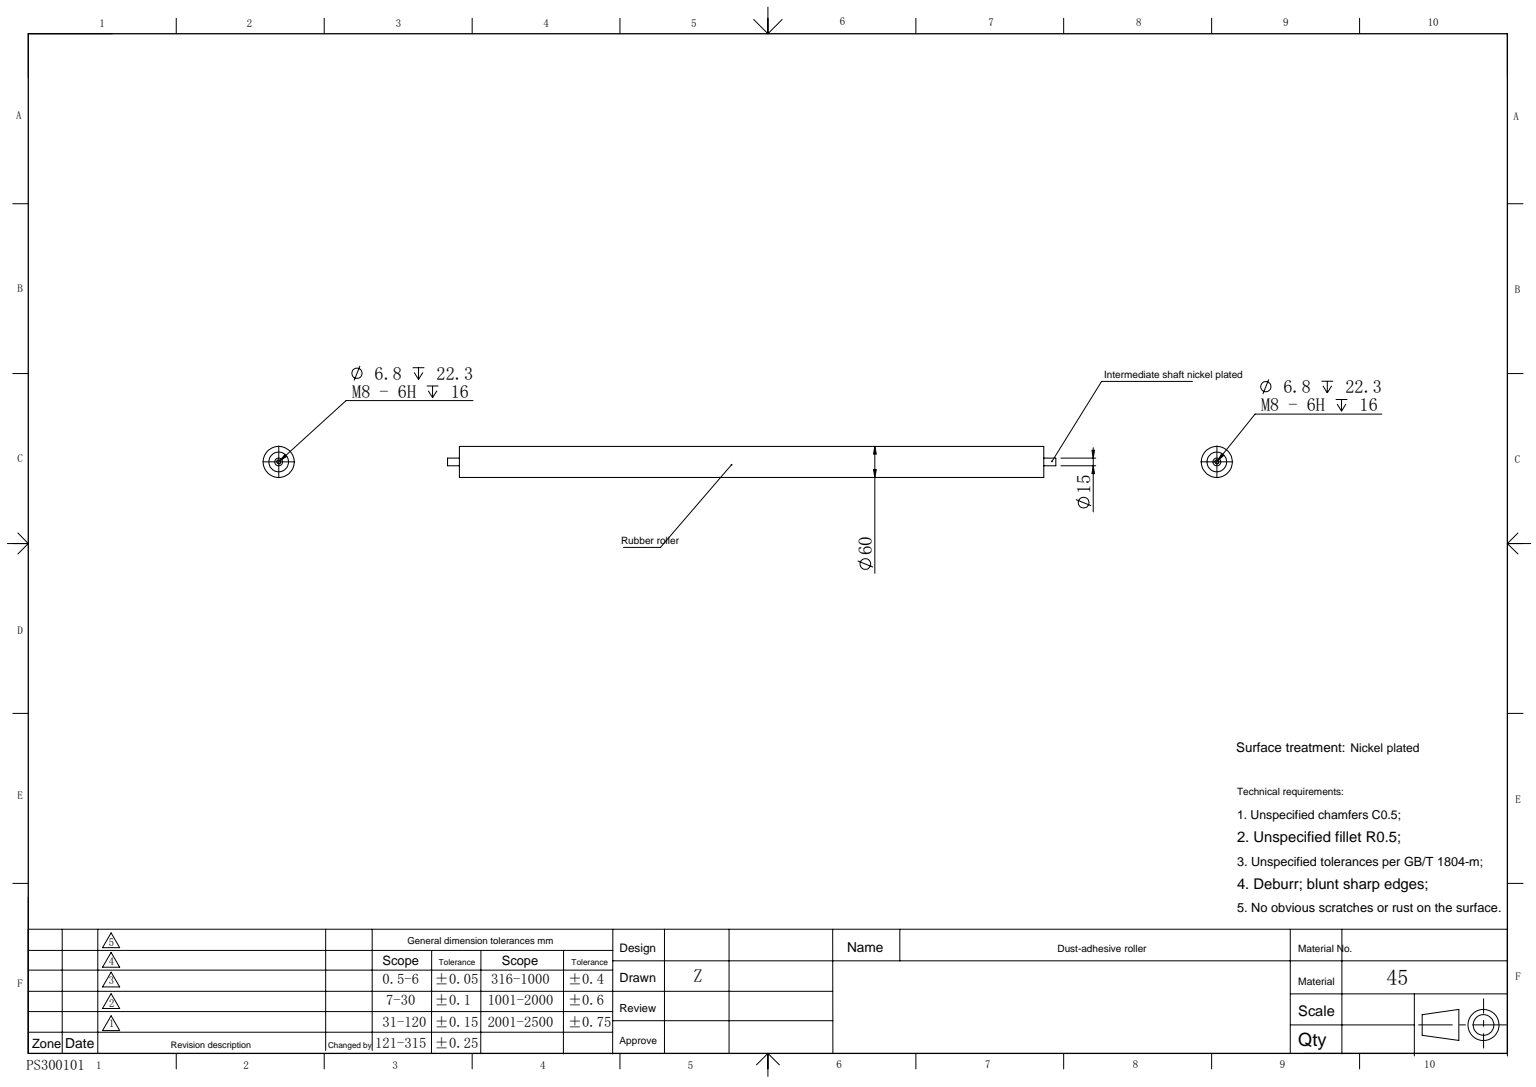
SolidWorks part; units mm, degrees
ref_plane "前视基准面" through (0, 0, 0) normal (0, 0, 1) x (1, 0, 0)
ref_plane "上视基准面" through (0, 0, 0) normal (0, 1, 0) x (1, 0, 0)
ref_plane "右视基准面" through (0, 0, 0) normal (1, 0, 0) x (0, 0, -1)
sketch "草图1" plane through (0, 0, 0) normal (0, 0, 1) x (1, 0, 0)
  circle A0 centre (0, 0) radius 7.5
  dimension "D1" = 15
extrude "凸台-拉伸1" add sketch "草图1" along normal mid plane 1176
sketch "草图2" plane through (0, 0, 0) normal (0, 0, 1) x (1, 0, 0)
  circle A0 centre (0, 0) radius 19
  dimension "D1" = 38
extrude "凸台-拉伸2" add sketch "草图2" along normal mid plane 1100
sketch "草图3" plane through (0, 0, 0) normal (0, 0, 1) x (1, 0, 0)
  circle A0 centre (0, 0) radius 30
  circle A1 centre (0, 0) radius 19
  circle A2 centre (0, 0) radius 19 construction
  dimension "D1" = 60
extrude "凸台-拉伸3" add sketch "草图3" along normal mid plane 1130 separate body
sketch "草图6" plane through (0, 0, -588) normal (0, 0, -1) x (-1, 0, 0)
  point P0 (0, 0)
hole_wizard "M8 螺纹孔1" positions "草图6" profile "草图5" tap size "M8" standard "ISO"
sketch "草图5" plane through (0, 0, -588) normal (1, 0, 0) x (0, 1, 0)
  line L0 (0, 0) -> (0, 24.2929)
  line L1 (0, 24.2929) -> (3.4, 22.25)
  line L2 (3.4, 22.25) -> (3.4, 0)
  line L5 (3.4, 0) -> (0, 0)
  line L10 (0, 24.2929) -> (-3.4, 22.25) construction
  line L11 (0, -6.35) -> (0, 107.95) construction
  dimension "螺纹孔钻头直径" = 6.8
  dimension "螺纹孔钻头深度" = 22.25
  dimension "导头角度" = 118
cosmetic thread "孔螺纹线1" parameters "D1"=16, "D2"=8
sketch "草图9" plane through (0, 0, 588) normal (0, 0, 1) x (1, 0, 0)
  point P0 (0, 0)
hole_wizard "M8 螺纹孔2" positions "草图9" profile "草图8" tap size "M8" standard "ISO"
sketch "草图8" plane through (0, 0, 588) normal (1, 0, 0) x (0, -1, 0)
  line L0 (0, 0) -> (0, 24.2929)
  line L1 (0, 24.2929) -> (3.4, 22.25)
  line L2 (3.4, 22.25) -> (3.4, 0)
  line L5 (3.4, 0) -> (0, 0)
  line L10 (0, 24.2929) -> (-3.4, 22.25) construction
  line L11 (0, -6.35) -> (0, 107.95) construction
  dimension "螺纹孔钻头直径" = 6.8
  dimension "螺纹孔钻头深度" = 22.25
  dimension "导头角度" = 118
cosmetic thread "孔螺纹线2" parameters "D1"=16, "D2"=8
